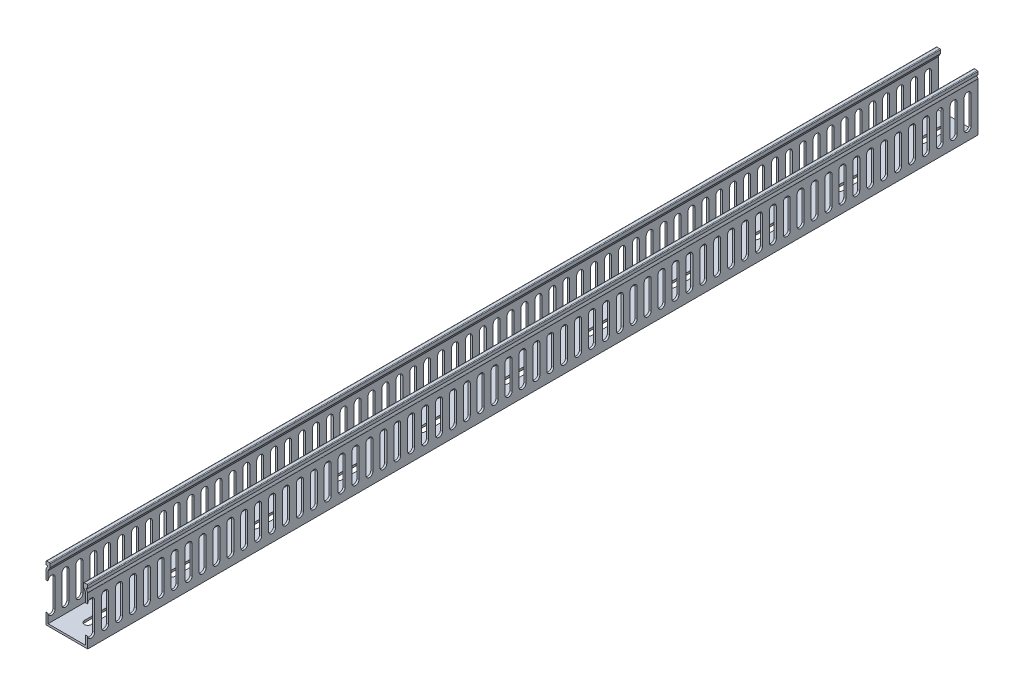
from build123d import *

# Parameters (mm, degrees)
EXTRUDE_1_DEPTH        = 640
CUT_EXTRUDE_2_DEPTH    = 642.950153828
PATTERN_LINEAR_1_COUNT = 130
PATTERN_LINEAR_1_PITCH = 10
CUT_EXTRUDE_3_DEPTH    = 642.424196613
PATTERN_LINEAR_2_COUNT = 25
PATTERN_LINEAR_2_PITCH = 60


with BuildPart() as part:
    # 草圖1 → 伸長1 (new body)
    with BuildSketch(Plane.XY):
        with BuildLine():
            Line((14.928746463, 35.118755895), (13.954348727, 36.742752122))
            ThreePointArc((13.954348727, 36.742752122), (13.947995236, 37.246349407), (14.383095189, 37.5))
            Line((14.383095189, 37.5), (15, 37.5))
            Line((15, 37.5), (15, 39.5))
            ThreePointArc((15, 39.5), (14.853553391, 39.853553391), (14.5, 40))
            Line((14.5, 40), (12.5, 40))
            ThreePointArc((12.5, 40), (12.146446609, 39.853553391), (12, 39.5))
            Line((12, 39.5), (12, 37.223016035))
            ThreePointArc((12, 37.223016035), (12.018142536, 37.089549244), (12.071253537, 36.965768157))
            Line((12.071253537, 36.965768157), (13.428746463, 34.703279948))
            ThreePointArc((13.428746463, 34.703279948), (13.481857464, 34.579498861), (13.5, 34.44603207))
            Line((13.5, 34.44603207), (13.5, 1.5))
            Line((13.5, 1.5), (-13.5, 1.5))
            Line((-13.5, 1.5), (-13.5, 34.44603207))
            ThreePointArc((-13.5, 34.44603207), (-13.481857464, 34.579498861), (-13.428746463, 34.703279948))
            Line((-13.428746463, 34.703279948), (-12.071253537, 36.965768157))
            ThreePointArc((-12.071253537, 36.965768157), (-12.018142536, 37.089549244), (-12, 37.223016035))
            Line((-12, 37.223016035), (-12, 39.5))
            ThreePointArc((-12, 39.5), (-12.146446609, 39.853553391), (-12.5, 40))
            Line((-12.5, 40), (-14.5, 40))
            ThreePointArc((-14.5, 40), (-14.853553391, 39.853553391), (-15, 39.5))
            Line((-15, 39.5), (-15, 37.5))
            Line((-15, 37.5), (-14.383095189, 37.5))
            ThreePointArc((-14.383095189, 37.5), (-13.947995236, 37.246349407), (-13.954348727, 36.742752122))
            Line((-13.954348727, 36.742752122), (-14.928746463, 35.118755895))
            ThreePointArc((-14.928746463, 35.118755895), (-14.981857464, 34.994974808), (-15, 34.861508018))
            Line((-15, 34.861508018), (-15, 0))
            Line((-15, 0), (15, 0))
            Line((15, 0), (15, 34.861508018))
            ThreePointArc((15, 34.861508018), (14.981857464, 34.994974808), (14.928746463, 35.118755895))
        make_face()
    extrude(amount=EXTRUDE_1_DEPTH)

    # 草圖2 → 伸長2 (cut, through all)
    with BuildSketch(Plane.ZY.offset(15)):
        with BuildLine():
            Line((5, 28), (5, 8))
            ThreePointArc((5, 8), (7.5, 5.5), (10, 8))
            Line((10, 8), (10, 28))
            ThreePointArc((10, 28), (7.5, 30.5), (5, 28))
        make_face()
    cut_extrude_2 = extrude(amount=-CUT_EXTRUDE_2_DEPTH, mode=Mode.SUBTRACT)

    # 直線複製排列1: 伸長2 ×130
    with Locations(*[(0, 0, i * PATTERN_LINEAR_1_PITCH) for i in range(1, PATTERN_LINEAR_1_COUNT)]):
        add(cut_extrude_2, mode=Mode.SUBTRACT)

    # 草圖3 → 伸長3 (cut, through all)
    with BuildSketch(Plane.XZ):
        with BuildLine():
            Line((-2.5, 25), (-2.5, 10))
            ThreePointArc((-2.5, 10), (0, 7.5), (2.5, 10))
            Line((2.5, 10), (2.5, 25))
            ThreePointArc((2.5, 25), (0, 27.5), (-2.5, 25))
        make_face()
    cut_extrude_3 = extrude(amount=-CUT_EXTRUDE_3_DEPTH, mode=Mode.SUBTRACT)

    # 直線複製排列2: 伸長3 ×25
    with Locations(*[(0, 0, i * PATTERN_LINEAR_2_PITCH) for i in range(1, PATTERN_LINEAR_2_COUNT)]):
        add(cut_extrude_3, mode=Mode.SUBTRACT)


solid = part.part
